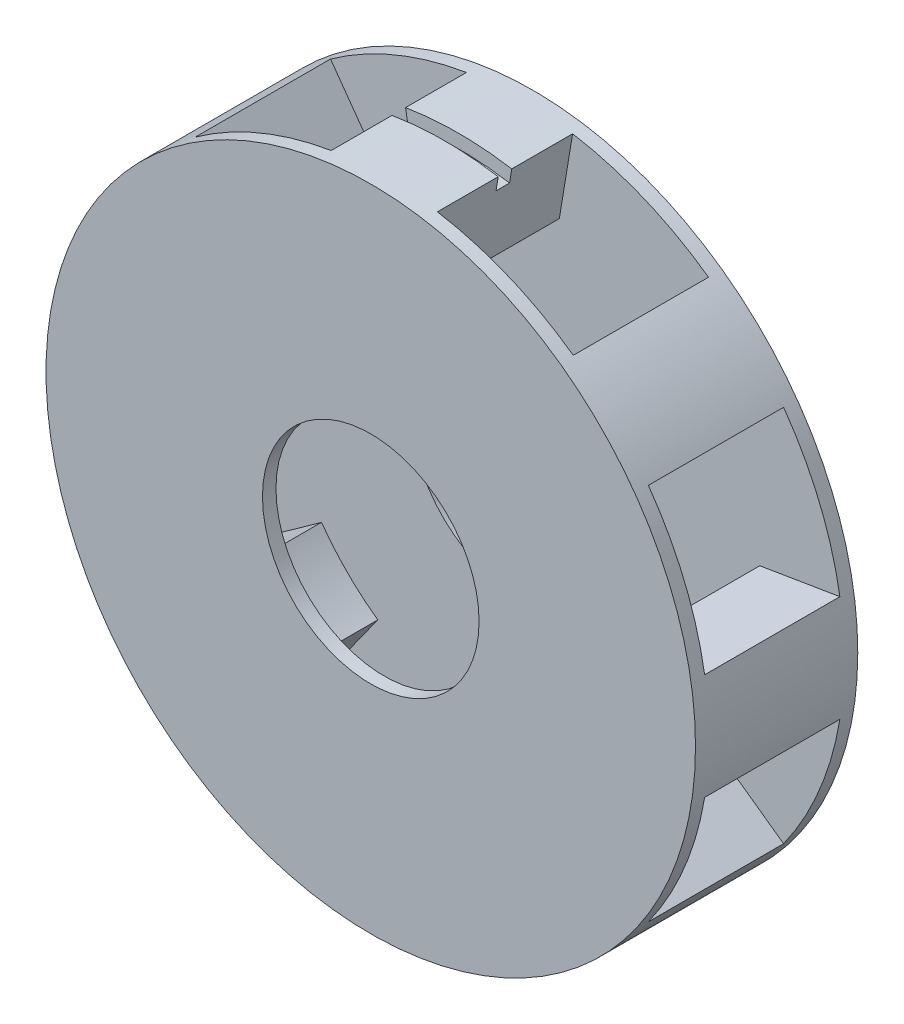
from build123d import *

# Parameters (mm, degrees)
SKETCH1_R           = 150
SKETCH1_R_2         = 120
BOSS_EXTRUDE1_DEPTH = 59.97
BOSS_EXTRUDE2_START = -59.97
SKETCH2_R           = 120
SKETCH2_R_2         = 90
BOSS_EXTRUDE2_DEPTH = 59.97
CUT_EXTRUDE1_START  = -59.97
CUT_EXTRUDE1_DEPTH  = 59.97
CIRPATTERN1_COUNT   = 8
CUT_EXTRUDE2_START  = -49.97
CUT_EXTRUDE2_DEPTH  = 49.97
CIRPATTERN2_COUNT   = 8
BOSS_EXTRUDE3_START = -5
SKETCH6_R           = 90
SKETCH6_R_2         = 40.03
BOSS_EXTRUDE3_DEPTH = 5
SKETCH7_R           = 90
SKETCH7_R_2         = 40.03
BOSS_EXTRUDE4_DEPTH = 5
SKETCH8_R           = 150
SKETCH8_R_2         = 120
CUT_EXTRUDE3_DEPTH  = 80
SKETCH10_W          = 5
SKETCH10_H          = 5
CUT_REVOLVE1_ANGLE  = 30


with BuildPart() as part:
    # Sketch1 → Boss-Extrude1 (new body)
    with BuildSketch(Plane.XY):
        Circle(SKETCH1_R)
        Circle(SKETCH1_R_2, mode=Mode.SUBTRACT)
    extrude(amount=BOSS_EXTRUDE1_DEPTH)

    # Sketch2 → Boss-Extrude2 (add)
    with BuildSketch(Plane.XY.offset(59.97).offset(BOSS_EXTRUDE2_START)):
        Circle(SKETCH2_R)
        Circle(SKETCH2_R_2, mode=Mode.SUBTRACT)
    extrude(amount=BOSS_EXTRUDE2_DEPTH)

    # Sketch3 → Cut-Extrude1 (cut)
    with BuildSketch(Plane.XY.offset(59.97).offset(CUT_EXTRUDE1_START)):
        with BuildLine():
            Line((-15.663143066, 118.973383365), (-19.578928833, 148.716729206))
            ThreePointArc((-19.578928833, 148.716729206), (0, 150), (19.578928833, 148.716729206))
            Line((19.578928833, 148.716729206), (15.663143066, 118.973383365))
            ThreePointArc((15.663143066, 118.973383365), (0, 120), (-15.663143066, 118.973383365))
        make_face()
    cut_extrude1 = extrude(amount=CUT_EXTRUDE1_DEPTH, mode=Mode.SUBTRACT)

    # CirPattern1: Cut-Extrude1 ×8 about axis
    cirpattern1_axis = Axis((0, 0, 0), (0, 0, 1))
    for i in range(1, CIRPATTERN1_COUNT):
        add(cut_extrude1.rotate(cirpattern1_axis, i * 360 / CIRPATTERN1_COUNT), mode=Mode.SUBTRACT)

    # Sketch5 → Cut-Extrude2 (cut)
    with BuildSketch(Plane.XY.offset(54.97).offset(CUT_EXTRUDE2_START)):
        with BuildLine():
            Line((14.714615406, 88.788963804), (24.524359011, 147.98160634))
            ThreePointArc((24.524359011, 147.98160634), (57.402514855, 138.581929877), (87.297456773, 121.980137895))
            Line((87.297456773, 121.980137895), (52.378474064, 73.188082737))
            ThreePointArc((52.378474064, 73.188082737), (34.441508913, 83.149157926), (14.714615406, 88.788963804))
        make_face()
    cut_extrude2 = extrude(amount=CUT_EXTRUDE2_DEPTH, mode=Mode.SUBTRACT)

    # CirPattern2: Cut-Extrude2 ×8 about axis
    cirpattern2_axis = Axis((0, 0, 0), (0, 0, 1))
    for i in range(1, CIRPATTERN2_COUNT):
        add(cut_extrude2.rotate(cirpattern2_axis, i * 360 / CIRPATTERN2_COUNT), mode=Mode.SUBTRACT)

    # Sketch6 → Boss-Extrude3 (add)
    with BuildSketch(Plane.XY.offset(59.97).offset(BOSS_EXTRUDE3_START)):
        Circle(SKETCH6_R)
        Circle(SKETCH6_R_2, mode=Mode.SUBTRACT)
    extrude(amount=BOSS_EXTRUDE3_DEPTH)

    # Sketch7 → Boss-Extrude4 (add)
    with BuildSketch(Plane(origin=(0, 0, 0), x_dir=(-1, 0, 0), z_dir=(0, 0, -1))):
        Circle(SKETCH7_R)
        with Locations(Location((0, 0, 0), (0, 0, 180))):
            Circle(SKETCH7_R_2, mode=Mode.SUBTRACT)
    extrude(amount=-BOSS_EXTRUDE4_DEPTH)

    # Sketch8 → Cut-Extrude3 (cut)
    with BuildSketch(Plane(origin=(0, 0, 0), x_dir=(-1, 0, 0), z_dir=(0, 0, -1))):
        Circle(SKETCH8_R)
        with Locations(Location((0, 0, 0), (0, 0, 180))):
            Circle(SKETCH8_R_2, mode=Mode.SUBTRACT)
    extrude(amount=-CUT_EXTRUDE3_DEPTH, mode=Mode.SUBTRACT)

    # Sketch10 → Cut-Revolve1 (revolve, cut)
    with BuildSketch(Plane(origin=(0, 0, 0), x_dir=(0, 0, -1), z_dir=(0.9865440422698816, -0.16349572673865878, 0))):
        with Locations((-29.985, 117.5)):
            Rectangle(SKETCH10_W, SKETCH10_H)
    revolve(axis=Axis((0, 0, 0), (0, 0, 1)), revolution_arc=CUT_REVOLVE1_ANGLE, mode=Mode.SUBTRACT)


solid = part.part
